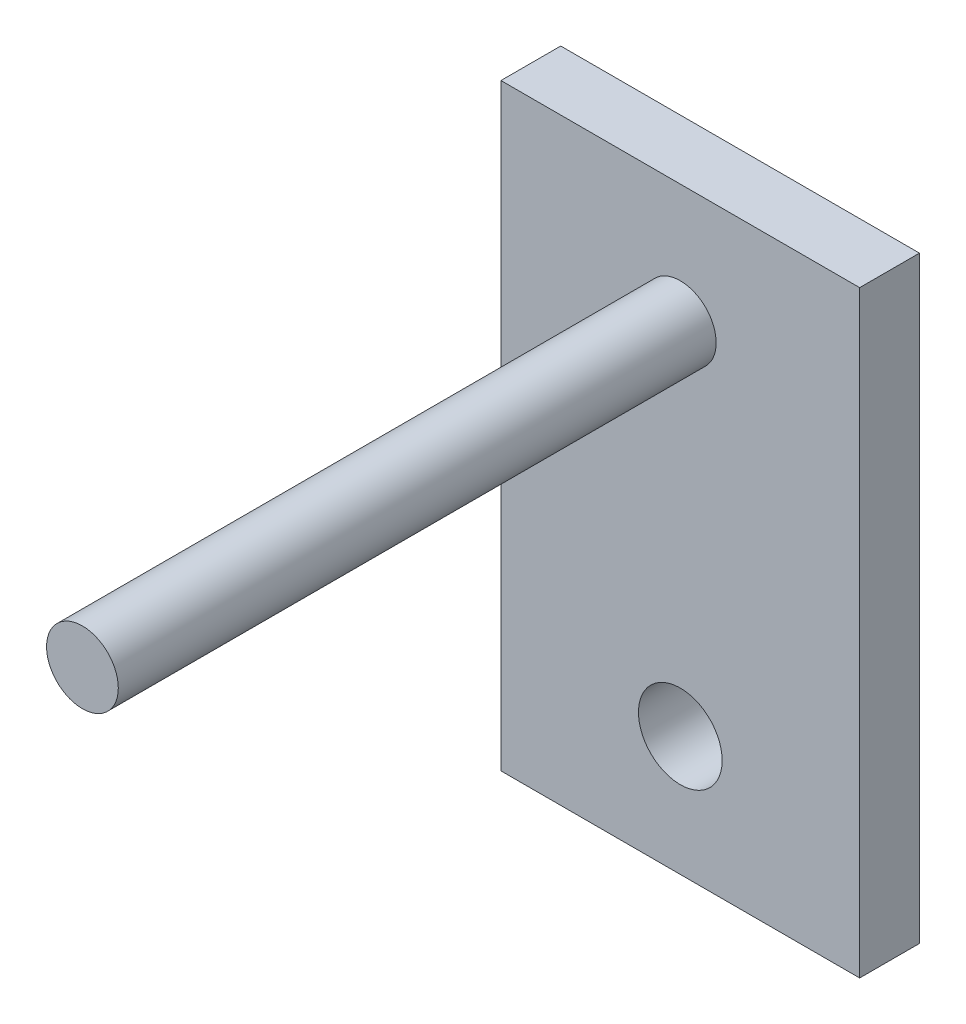
from build123d import *

# Parameters (mm, degrees)
SKETCH1_W           = 60
SKETCH1_H           = 100
SKETCH1_R           = 7
BOSS_EXTRUDE1_DEPTH = 10
SKETCH2_R           = 6
BOSS_EXTRUDE2_DEPTH = 100


with BuildPart() as part:
    # Sketch1 → Boss-Extrude1 (new body)
    with BuildSketch(Plane.XY):
        Rectangle(SKETCH1_W, SKETCH1_H)
        with Locations((0, -30)):
            Circle(SKETCH1_R, mode=Mode.SUBTRACT)
    extrude(amount=BOSS_EXTRUDE1_DEPTH)

    # Sketch2 → Boss-Extrude2 (add)
    with BuildSketch(Plane.XY.offset(10)):
        with Locations(Location((0, 30, 0), (0, 0, 180))):
            Circle(SKETCH2_R)
    extrude(amount=BOSS_EXTRUDE2_DEPTH)


solid = part.part
